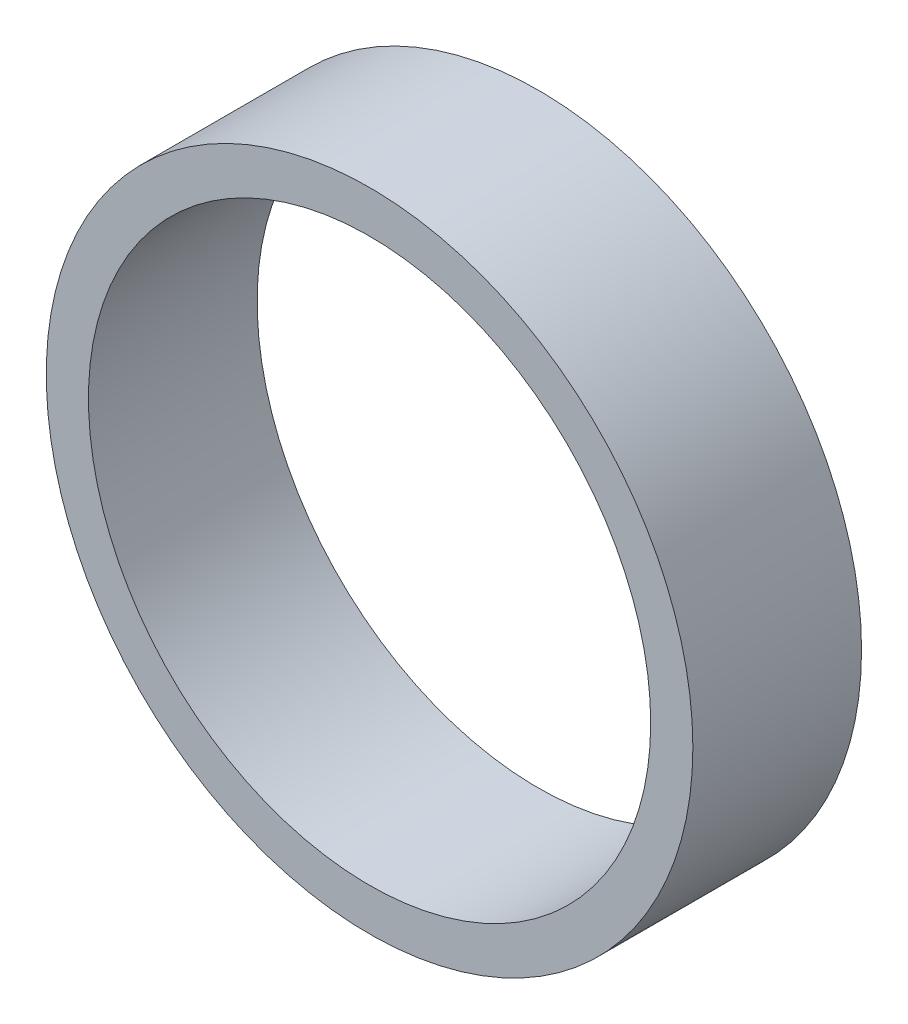
from build123d import *

# Parameters (mm, degrees)
SKETCH_1_R      = 23
SKETCH_1_R_2    = 20
EXTRUDE_1_DEPTH = 12


with BuildPart() as part:
    # 草图1 → 凸台-拉伸1 (new body)
    with BuildSketch(Plane.XY):
        Circle(SKETCH_1_R)
        Circle(SKETCH_1_R_2, mode=Mode.SUBTRACT)
    extrude(amount=EXTRUDE_1_DEPTH)


solid = part.part
